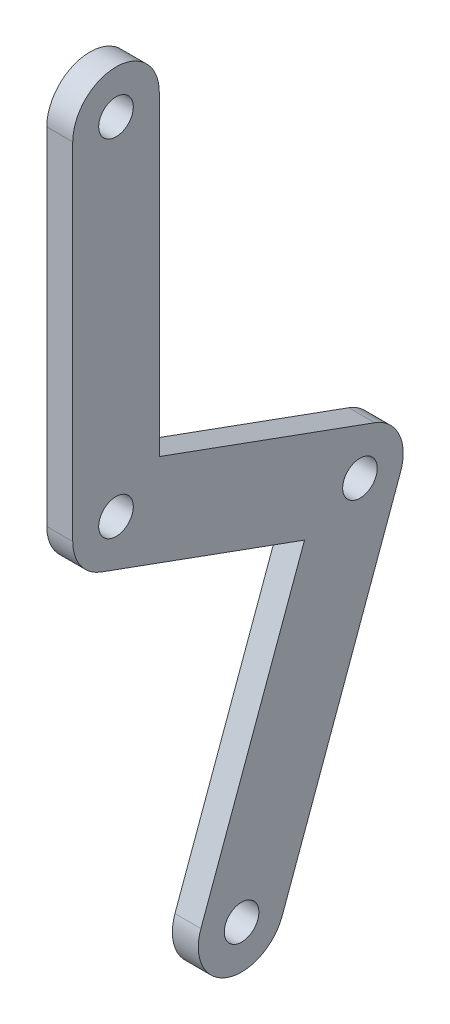
from build123d import *

# Parameters (mm, degrees)
SKETCH1_R           = 4
BOSS_EXTRUDE1_DEPTH = 6


with BuildPart() as part:
    # Sketch1 → Boss-Extrude1 (new body)
    # profile 1 of 5: a face of its own
    with BuildSketch(Plane(origin=(0, 0, 0), x_dir=(0, 0, -1), z_dir=(1, 0, 0))):
        with BuildLine():
            Line((38.416871989, -99.116819696), (65.778483455, -23.941410033))
            ThreePointArc((65.778483455, -23.941410033), (60.607739865, -29.58428647), (52.961355814, -29.918134807))
            Line((52.961355814, -29.918134807), (43.564429606, -26.497933374))
            Line((43.564429606, -26.497933374), (19.623019573, -92.276416829))
            ThreePointArc((19.623019573, -92.276416829), (25.599744348, -105.09354447), (38.416871989, -99.116819696))
        make_face()
        with Locations((29.019945781, -95.696618262)):
            Circle(SKETCH1_R, mode=Mode.SUBTRACT)
    # profile 2 of 5: a face of its own
    with BuildSketch(Plane(origin=(0, 0, 0), x_dir=(0, 0, -1), z_dir=(1, 0, 0))):
        with BuildLine():
            ThreePointArc((65.778483455, -23.941410033), (65.444635118, -16.295025982), (59.80175868, -11.124282392))
            ThreePointArc((59.80175868, -11.124282392), (52.15537463, -11.458130729), (46.984631039, -17.101007166))
            Line((46.984631039, -17.101007166), (43.564429606, -26.497933374))
            Line((43.564429606, -26.497933374), (52.961355814, -29.918134807))
            ThreePointArc((52.961355814, -29.918134807), (60.607739865, -29.58428647), (65.778483455, -23.941410033))
        make_face()
        with Locations((56.381557247, -20.5212086)):
            Circle(SKETCH1_R, mode=Mode.SUBTRACT)
    # profile 3 of 5: a face of its own
    with BuildSketch(Plane(origin=(0, 0, 0), x_dir=(0, 0, -1), z_dir=(1, 0, 0))):
        with BuildLine():
            Line((59.80175868, -11.124282392), (10, 7.002075382))
            Line((10, 7.002075382), (10, 0))
            ThreePointArc((10, 0), (5.735764364, -8.191520443), (-3.420201433, -9.396926208))
            Line((-3.420201433, -9.396926208), (43.564429606, -26.497933374))
            Line((43.564429606, -26.497933374), (46.984631039, -17.101007166))
            ThreePointArc((46.984631039, -17.101007166), (52.15537463, -11.458130729), (59.80175868, -11.124282392))
        make_face()
    # profile 4 of 5: a face of its own
    with BuildSketch(Plane(origin=(0, 0, 0), x_dir=(0, 0, -1), z_dir=(1, 0, 0))):
        with BuildLine():
            Line((10, 0), (10, 7.002075382))
            Line((10, 7.002075382), (3.420201433, 9.396926208))
            ThreePointArc((3.420201433, 9.396926208), (-5.735764364, 8.191520443), (-10, 0))
            ThreePointArc((-10, 0), (-8.191520443, -5.735764364), (-3.420201433, -9.396926208))
            ThreePointArc((-3.420201433, -9.396926208), (5.735764364, -8.191520443), (10, 0))
        make_face()
        Circle(SKETCH1_R, mode=Mode.SUBTRACT)
    # profile 5 of 5: a face of its own
    with BuildSketch(Plane(origin=(0, 0, 0), x_dir=(0, 0, -1), z_dir=(1, 0, 0))):
        with BuildLine():
            Line((10, 7.002075382), (10, 80))
            ThreePointArc((10, 80), (0, 90), (-10, 80))
            Line((-10, 80), (-10, 0))
            ThreePointArc((-10, 0), (-5.735764364, 8.191520443), (3.420201433, 9.396926208))
            Line((3.420201433, 9.396926208), (10, 7.002075382))
        make_face()
        with Locations((0, 80)):
            Circle(SKETCH1_R, mode=Mode.SUBTRACT)
    extrude(amount=BOSS_EXTRUDE1_DEPTH)


solid = part.part
